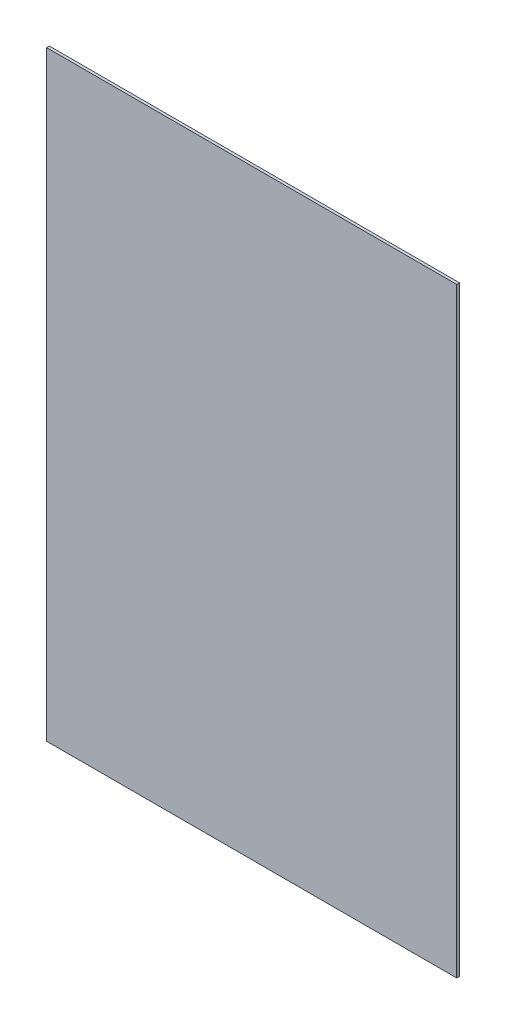
SolidWorks part; units mm, degrees
material "PMMA(有机玻璃)"
ref_plane "前视" through (0, 0, 0) normal (0, 0, 1) x (1, 0, 0)
ref_plane "上视" through (0, 0, 0) normal (0, 1, 0) x (1, 0, 0)
ref_plane "右视" through (0, 0, 0) normal (1, 0, 0) x (0, 0, -1)
sketch "草图1" plane through (0, 0, 0) normal (0, 0, 1) x (1, 0, 0)
  line L1 (-372.5, 545.5) -> (372.5, 545.5)
  line L2 (-372.5, 545.5) -> (-372.5, -545.5)
  line L3 (-372.5, -545.5) -> (372.5, -545.5)
  line L4 (372.5, 545.5) -> (372.5, -545.5)
  line L5 (-372.5, 545.5) -> (372.5, -545.5) construction
  line L6 (-372.5, -545.5) -> (372.5, 545.5) construction
  point P0 (0, 0)
  dimension "D1" = 1091
  dimension "D2" = 745
extrude "凸台-拉伸1" add sketch "草图1" along normal blind 5
hole_wizard "M5 间隙孔1" positions "草图3" profile "草图2" hole size "M5" standard "GB"
sketch "草图3" plane through (0, 0, 5) normal (0, 0, 1) x (1, 0, 0)
  line L0 (-427.5, 273) -> (-427.5, -273) construction
  line L1 (-427.5, -273) -> (427.5, -273) construction
  line L2 (0, 273) -> (0, -273) construction
  line L3 (427.5, 273) -> (-427.5, 273) construction
  line L5 (-427.5, 0) -> (427.5, 0) construction
  line L6 (427.5, -273) -> (427.5, 273) construction
  point P0 (-375, -261)
  point P46 (415.5, 250)
  point P48 (-415.5, 250)
  point P58 (-125, -261)
  point P59 (125, -261)
  point P61 (-125, 261)
  point P62 (125, 261)
  point P64 (-375, 261)
  point P88 (375, -261)
  point P89 (375, 261)
  point P108 (415.5, 0)
  point P109 (-415.5, 0)
  point P110 (415.5, -250)
  point P111 (-415.5, -250)
  dimension "D1" = 12
  dimension "D2" = 12
  dimension "D5" = 3
  dimension "D3" = 12
  dimension "D6" = 4
  dimension "D4" = 2
sketch "草图2" plane through (-375, -261, 5) normal (1, 0, 0) x (0, -1, 0)
  line L0 (0, 0) -> (0, 5)
  line L1 (0, 5) -> (2.75, 5)
  line L2 (2.75, 5) -> (2.75, 0)
  line L5 (2.75, 0) -> (0, 0)
  line L11 (0, -6.35) -> (0, 107.95) construction
  dimension "通孔孔直径" = 5.5
  dimension "通孔孔深度" = 5
